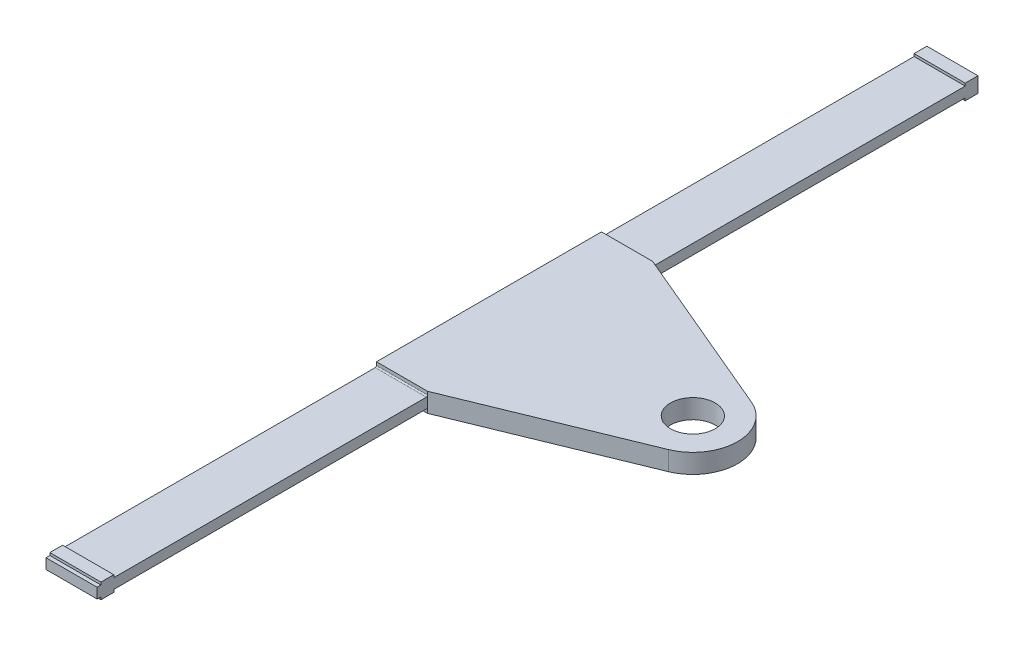
SolidWorks part; units mm, degrees
ref_plane "前视基准面" through (0, 0, 0) normal (0, 0, 1) x (1, 0, 0)
ref_plane "上视基准面" through (0, 0, 0) normal (0, 1, 0) x (1, 0, 0)
ref_plane "右视基准面" through (0, 0, 0) normal (1, 0, 0) x (0, 0, -1)
other "Configuration Table"
sketch "草图1" plane through (0, 0, 0) normal (0, 0, 1) x (1, 0, 0)
  line L1 (-20, -4) -> (20, -4)
  line L2 (-20, -4) -> (-20, 4)
  line L3 (-20, 4) -> (20, 4)
  line L4 (20, -4) -> (20, 4)
  line L5 (-20, -4) -> (20, 4) construction
  line L6 (-20, 4) -> (20, -4) construction
  point P0 (0, 0)
  dimension "D1" = 40
  dimension "D2" = 8
extrude "凸台-拉伸1" add sketch "草图1" along normal mid plane 661
sketch "草图6" plane through (0, 0, -330.5) normal (0, 0, -1) x (-1, 0, 0)
  line L4 (-20, 4) -> (-20, -4)
  line L5 (-20, -4) -> (20, -4)
  line L6 (20, -4) -> (20, 4)
  line L7 (20, 4) -> (-20, 4)
  line L8 (-20, 4) -> (-20, -4)
  line L9 (-20, -4) -> (20, -4)
  line L10 (20, -4) -> (20, 4)
  line L11 (20, 4) -> (-20, 4)
  dimension "D1" = 0
sketch "草图7" plane through (0, 0, -330.5) normal (0, 0, -1) x (-1, 0, 0)
  line L4 (-20, 4) -> (-20, -4)
  line L5 (-20, -4) -> (20, -4)
  line L6 (20, -4) -> (20, 4)
  line L7 (20, 4) -> (-20, 4)
  line L8 (-20, 4) -> (-20, -4)
  line L9 (-20, -4) -> (20, -4)
  line L10 (20, -4) -> (20, 4)
  line L11 (20, 4) -> (-20, 4)
  dimension "D1" = 0
sketch "草图13" plane through (0, -4, 0) normal (0, -1, 0) x (1, 0, 0)
  line L0 (153.6222, 33.3043) -> (20, 88)
  line L1 (20, 330.5) -> (20, -330.5) construction
  line L2 (153.9981, -31.3221) -> (20, -88)
  line L3 (20, 88) -> (20, -88)
  arc A0 (153.9981, -31.3221) -> (153.6222, 33.3043) centre (140.3635, 0.9129) ccw
  dimension "D1" = 70
  dimension "D2" = 88
  dimension "D3" = 88
extrude "凸台-拉伸9" add sketch "草图13" along normal mid plane 15 from offset 4 offset against normal yes
sketch "草图14" plane through (0, -7.5, 0) normal (0, -1, 0) x (1, 0, 0)
  circle A0 centre (140.3635, 0.9129) radius 17.5
  dimension "D1" = 35
extrude "切除-拉伸1" cut sketch "草图14" against normal through all both and the other way through all
sketch "草图15" plane through (-20, 0, 0) normal (-1, 0, 0) x (0, 0, 1)
  line L0 (330.5, 4) -> (333.5, 4)
  line L3 (330.5, -4) -> (330.5, 4)
  line L5 (333.5, -6) -> (343.5, -6)
  line L6 (333.5, -6) -> (333.5, -4)
  line L7 (333.5, 6) -> (343.5, 6)
  line L10 (346.5, 0.5169) -> (346.5, -4)
  line L12 (333.5, 4) -> (333.5, 6)
  line L13 (330.5, 0) -> (338.5, 0) construction
  line L14 (333.5, -4) -> (330.5, -4)
  line L15 (346.5, 0.5169) -> (346.5, 4)
  line L16 (343.5, -6) -> (343.5, -4)
  line L17 (343.5, 4) -> (346.5, 4)
  line L19 (343.5, -4) -> (346.5, -4)
  line L20 (343.5, 4) -> (343.5, 6)
  line L21 (343.5, 0) -> (353.0074, 0) construction
  point P3 (338.5, 0)
  dimension "D1" = 6
  dimension "D3" = 3
  dimension "D4" = 6
  dimension "D5" = 3
extrude "凸台-拉伸10" add sketch "草图15" against normal up to surface (40 mm away) up to face at (20, 0, 209.25)
sketch "草图16" plane through (20, 0, 0) normal (-1, 0, 0) x (0, 0, 1)
  line L4 (-88, 4) -> (88, 4)
  line L5 (88, 4) -> (88, 7.5)
  line L6 (88, 7.5) -> (-88, 7.5)
  line L7 (-88, 7.5) -> (-88, 4)
  line L8 (-88, 4) -> (88, 4)
  line L9 (88, 4) -> (88, 7.5)
  line L10 (88, 7.5) -> (-88, 7.5)
  line L11 (-88, 7.5) -> (-88, 4)
  dimension "D1" = 0
extrude "凸台-拉伸11" add sketch "草图16" along normal up to surface (40 mm away) up to face at (-20, 0, 228.3333)
sketch "草图17" plane through (20, 0, 0) normal (-1, 0, 0) x (0, 0, 1)
  line L4 (88, -7.5) -> (88, -4)
  line L5 (88, -4) -> (-88, -4)
  line L6 (-88, -4) -> (-88, -7.5)
  line L7 (-88, -7.5) -> (88, -7.5)
  line L8 (88, -7.5) -> (88, -4)
  line L9 (88, -4) -> (-88, -4)
  line L10 (-88, -4) -> (-88, -7.5)
  line L11 (-88, -7.5) -> (88, -7.5)
  dimension "D1" = 0
extrude "凸台-拉伸12" add sketch "草图17" along normal up to surface (40 mm away) up to face at (-20, 1.4375, 171.25)
mirror "镜向1" about plane through (0, 0, 0) normal (0, 0, 1) of "凸台-拉伸10"
fillet "圆角1" radius 1 4 edges at (0, 4, 88) (0, 4, -88) (0, -4, -88) (0, -4, 88)
sketch "草图18" plane through (-20, 0, 0) normal (-1, 0, 0) x (0, 0, 1)
  line L0 (-339.5, 6) -> (-339.5, 4)
  line L1 (-339.5, 4) -> (-342.5, 4)
  line L2 (-342.5, 4) -> (-342.5, -4)
  line L3 (-342.5, -4) -> (-339.5, -4)
  line L4 (-339.5, -4) -> (-339.5, -6)
  line L28 (-88, 7.5) -> (-88, 5)
  line L29 (-89, 4) -> (-333.5, 4)
  line L30 (-333.5, 4) -> (-333.5, 6)
  line L31 (-333.5, 6) -> (-343.5, 6)
  line L32 (-343.5, 6) -> (-343.5, 4)
  line L33 (-343.5, 4) -> (-346.5, 4)
  line L34 (-346.5, 4) -> (-346.5, -4)
  line L35 (-346.5, -4) -> (-343.5, -4)
  line L36 (-343.5, -4) -> (-343.5, -6)
  line L37 (-343.5, -6) -> (-333.5, -6)
  line L38 (-333.5, -6) -> (-333.5, -4)
  line L39 (-333.5, -4) -> (-89, -4)
  line L40 (-88, -5) -> (-88, -7.5)
  line L41 (-88, -7.5) -> (88, -7.5)
  line L42 (88, -7.5) -> (88, -5)
  line L43 (89, -4) -> (333.5, -4)
  line L44 (333.5, -4) -> (333.5, -6)
  line L45 (333.5, -6) -> (343.5, -6)
  line L46 (343.5, -6) -> (343.5, -4)
  line L47 (343.5, -4) -> (346.5, -4)
  line L48 (346.5, -4) -> (346.5, 4)
  line L49 (346.5, 4) -> (343.5, 4)
  line L50 (343.5, 4) -> (343.5, 6)
  line L51 (343.5, 6) -> (333.5, 6)
  line L52 (333.5, 6) -> (333.5, 4)
  line L53 (333.5, 4) -> (89, 4)
  line L54 (88, 5) -> (88, 7.5)
  line L55 (88, 7.5) -> (-88, 7.5)
  line L56 (-88, 7.5) -> (-88, 5)
  line L59 (-339.5, 6) -> (-343.5, 6)
  line L60 (-343.5, 6) -> (-343.5, 4)
  line L61 (-343.5, 4) -> (-346.5, 4)
  line L62 (-346.5, 4) -> (-346.5, -4)
  line L63 (-346.5, -4) -> (-343.5, -4)
  line L64 (-343.5, -4) -> (-343.5, -6)
  line L65 (-343.5, -6) -> (-339.5, -6)
  line L68 (-88, -5) -> (-88, -7.5)
  line L69 (-88, -7.5) -> (88, -7.5)
  line L70 (88, -7.5) -> (88, -5)
  line L71 (89, -4) -> (333.5, -4)
  line L72 (333.5, -4) -> (333.5, -6)
  line L73 (333.5, -6) -> (343.5, -6)
  line L74 (343.5, -6) -> (343.5, -4)
  line L75 (343.5, -4) -> (346.5, -4)
  line L76 (346.5, -4) -> (346.5, 4)
  line L77 (346.5, 4) -> (343.5, 4)
  line L78 (343.5, 4) -> (343.5, 6)
  line L79 (343.5, 6) -> (333.5, 6)
  line L80 (333.5, 6) -> (333.5, 4)
  line L81 (333.5, 4) -> (89, 4)
  line L82 (88, 5) -> (88, 7.5)
  line L83 (88, 7.5) -> (-88, 7.5)
  arc A4 (-89, 4) -> (-88, 5) centre (-89, 5) ccw
  arc A5 (-88, -5) -> (-89, -4) centre (-89, -5) ccw
  arc A6 (89, -4) -> (88, -5) centre (89, -5) ccw
  arc A7 (88, 5) -> (89, 4) centre (89, 5) ccw
  arc A8 (-89, 4) -> (-88, 5) centre (-89, 5) ccw
  arc A9 (-88, -5) -> (-89, -4) centre (-89, -5) ccw
  arc A10 (89, -4) -> (88, -5) centre (89, -5) ccw
  arc A11 (88, 5) -> (89, 4) centre (89, 5) ccw
  line M40 (-333.5, 6) -> (-343.5, 6)
  line M41 (-343.5, 6) -> (-343.5, 4)
  line M42 (-343.5, 4) -> (-346.5, 4)
  line M43 (-346.5, 4) -> (-346.5, -4)
  line M44 (-346.5, -4) -> (-343.5, -4)
  line M45 (-343.5, -4) -> (-343.5, -6)
  line M46 (-343.5, -6) -> (-333.5, -6)
  dimension "D2" = 4
  dimension "D3" = 3
  dimension "D4" = 3
  dimension "D1" = 0
extrude "切除-拉伸2" cut sketch "草图18" against normal through all both and the other way through all contours L4 L3 L2 L1 L0 M40 M41 M42 M43 M44 M45 M46
sketch "草图19" plane through (-20, 0, 0) normal (-1, 0, 0) x (0, 0, 1)
  line L0 (-332.5, 4) -> (-332.5, 6)
  line L1 (-332.5, 6) -> (-342.5, 6)
  line L2 (-342.5, 6) -> (-342.5, -6)
  line L3 (-342.5, -6) -> (-332.5, -6)
  line L4 (-332.5, -6) -> (-332.5, -4)
  line L6 (-332.5, 4) -> (-332.5, -4)
  line L28 (-339.5, -4) -> (-339.5, -6)
  line L29 (-339.5, -6) -> (-333.5, -6)
  line L30 (-333.5, -6) -> (-333.5, -4)
  line L31 (-333.5, -4) -> (-89, -4)
  line L32 (-88, -5) -> (-88, -7.5)
  line L33 (-88, -7.5) -> (88, -7.5)
  line L34 (88, -7.5) -> (88, -5)
  line L35 (89, -4) -> (333.5, -4)
  line L36 (333.5, -4) -> (333.5, -6)
  line L37 (333.5, -6) -> (343.5, -6)
  line L38 (343.5, -6) -> (343.5, -4)
  line L39 (343.5, -4) -> (346.5, -4)
  line L40 (346.5, -4) -> (346.5, 4)
  line L41 (346.5, 4) -> (343.5, 4)
  line L42 (343.5, 4) -> (343.5, 6)
  line L43 (343.5, 6) -> (333.5, 6)
  line L44 (333.5, 6) -> (333.5, 4)
  line L45 (333.5, 4) -> (89, 4)
  line L46 (88, 5) -> (88, 7.5)
  line L47 (88, 7.5) -> (-88, 7.5)
  line L48 (-88, 7.5) -> (-88, 5)
  line L49 (-89, 4) -> (-333.5, 4)
  line L50 (-333.5, 4) -> (-333.5, 6)
  line L51 (-333.5, 6) -> (-339.5, 6)
  line L52 (-339.5, 6) -> (-339.5, 4)
  line L53 (-339.5, 4) -> (-342.5, 4)
  line L54 (-342.5, 4) -> (-342.5, -4)
  line L55 (-342.5, -4) -> (-339.5, -4)
  line L57 (-339.5, -6) -> (-333.5, -6)
  line L60 (-88, -5) -> (-88, -7.5)
  line L61 (-88, -7.5) -> (88, -7.5)
  line L62 (88, -7.5) -> (88, -5)
  line L63 (89, -4) -> (333.5, -4)
  line L64 (333.5, -4) -> (333.5, -6)
  line L65 (333.5, -6) -> (343.5, -6)
  line L66 (343.5, -6) -> (343.5, -4)
  line L67 (343.5, -4) -> (346.5, -4)
  line L68 (346.5, -4) -> (346.5, 4)
  line L69 (346.5, 4) -> (343.5, 4)
  line L70 (343.5, 4) -> (343.5, 6)
  line L71 (343.5, 6) -> (333.5, 6)
  line L72 (333.5, 6) -> (333.5, 4)
  line L73 (333.5, 4) -> (89, 4)
  line L74 (88, 5) -> (88, 7.5)
  line L75 (88, 7.5) -> (-88, 7.5)
  line L76 (-88, 7.5) -> (-88, 5)
  line L79 (-333.5, 6) -> (-339.5, 6)
  line L82 (-342.5, 4) -> (-342.5, -4)
  arc A4 (-88, -5) -> (-89, -4) centre (-89, -5) ccw
  arc A5 (89, -4) -> (88, -5) centre (89, -5) ccw
  arc A6 (88, 5) -> (89, 4) centre (89, 5) ccw
  arc A7 (-89, 4) -> (-88, 5) centre (-89, 5) ccw
  arc A8 (-88, -5) -> (-89, -4) centre (-89, -5) ccw
  arc A9 (89, -4) -> (88, -5) centre (89, -5) ccw
  arc A10 (88, 5) -> (89, 4) centre (89, 5) ccw
  arc A11 (-89, 4) -> (-88, 5) centre (-89, 5) ccw
  dimension "D1" = 0
extrude "凸台-拉伸13" add sketch "草图19" against normal up to surface (40 mm away) contours L0 L1 L2 L3 L4 L6 up to face at (20, 0, -266.4704)
